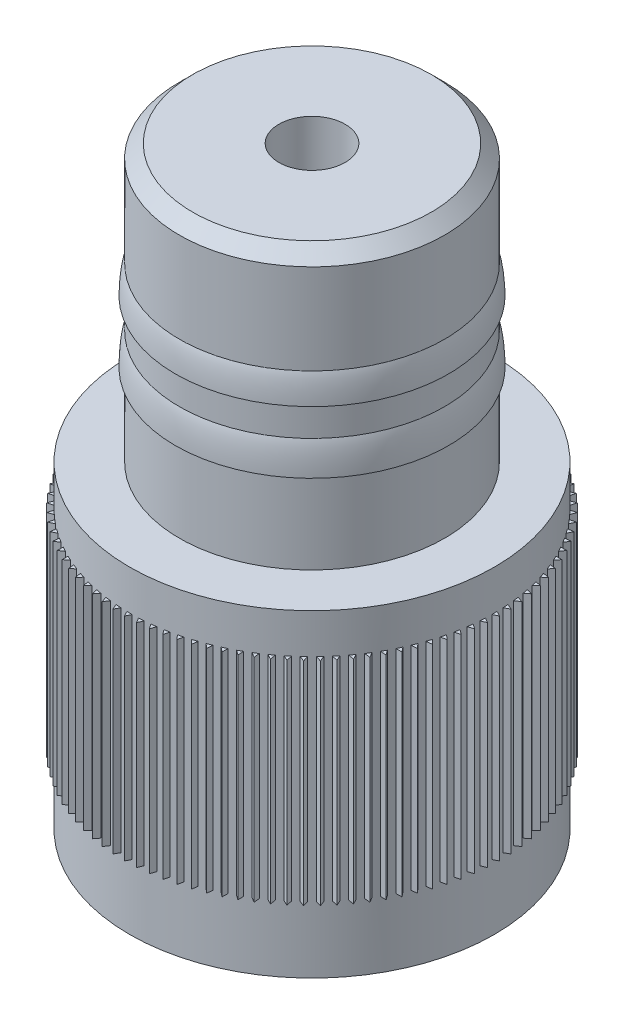
from build123d import *

# Parameters (mm, degrees)
CHAMFER1_SIZE       = 0.5
BOSS_EXTRUDE1_START = -8
BOSS_EXTRUDE1_DEPTH = 8
CIRPATTERN1_COUNT   = 100


with BuildPart() as part:
    # Sketch1 → Revolve1 (revolve)
    with BuildSketch(Plane.XY, mode=Mode.PRIVATE) as revolve1_sk:
        with BuildLine():
            Line((-5, 0), (-5, 3.1))
            Line((-5, 3.1), (-5.15, 3.1))
            add(Edge.make_bspline(
                [(-5, 4.297032053), (-5.05121173, 4.142122175), (-5.086517142, 3.960249608), (-5.134772947, 3.550843087), (-5.146982855, 3.330472207), (-5.15, 3.1)],
                knots=[0, 0, 0, 0, 0.5, 0.5, 1, 1, 1, 1], degree=3))
            Line((-5, 4.297032053), (-5, 5.440840859))
            Line((-5, 5.440840859), (-5.15, 5.440840859))
            add(Edge.make_bspline(
                [(-5, 6.5), (-5.047605665, 6.363384357), (-5.0814919, 6.202637521), (-5.130093219, 5.840342723), (-5.144049999, 5.645135031), (-5.15, 5.440840859)],
                knots=[0, 0, 0, 0, 0.5, 0.5, 1, 1, 1, 1], degree=3))
            Line((-5, 6.5), (-5, 10.4))
            Line((-5, 10.4), (-1.25, 10.4))
            Line((-1.25, 10.4), (-1.25, 0))
            Line((-1.25, 0), (-2.525, 0))
            Line((-2.525, 0), (-2.525, -8.44))
            Line((-2.525, -8.44), (-2.725, -8.44))
            Line((-2.725, -8.44), (-2.725, 0))
            Line((-2.725, 0), (-3.225, 0))
            Line((-3.225, 0), (-3.225, -12))
            Line((-3.225, -12), (-6.88, -12))
            Line((-6.88, -12), (-6.88, 0))
            Line((-6.88, 0), (-5, 0))
        make_face()
    revolve(revolve1_sk.sketch.rotate(Axis((0, -30.576267402, 0), (0, 1, 0)), 270), axis=Axis((0, -30.576267402, 0), (0, 1, 0)))

    # Chamfer1
    chamfer1_edges = [part.edges().sort_by_distance(p)[0] for p in [
        (0, 10.4, 5),
    ]]
    chamfer(chamfer1_edges, length=CHAMFER1_SIZE)

    # Sketch2 → Boss-Extrude1 (add)
    with BuildSketch(Plane.XZ.offset(9.5).offset(BOSS_EXTRUDE1_START)):
        with BuildLine():
            Line((0, 7.08), (-0.1, 6.879273217))
            ThreePointArc((-0.1, 6.879273217), (0, 6.88), (0.1, 6.879273217))
            Line((0.1, 6.879273217), (0, 7.08))
        make_face()
    boss_extrude1 = extrude(amount=BOSS_EXTRUDE1_DEPTH)

    # CirPattern1: Boss-Extrude1 ×100 about axis
    cirpattern1_axis = Axis((0, 0, 0), (0, 1, 0))
    for i in range(1, CIRPATTERN1_COUNT):
        add(boss_extrude1.rotate(cirpattern1_axis, i * 360 / CIRPATTERN1_COUNT))


solid = part.part
